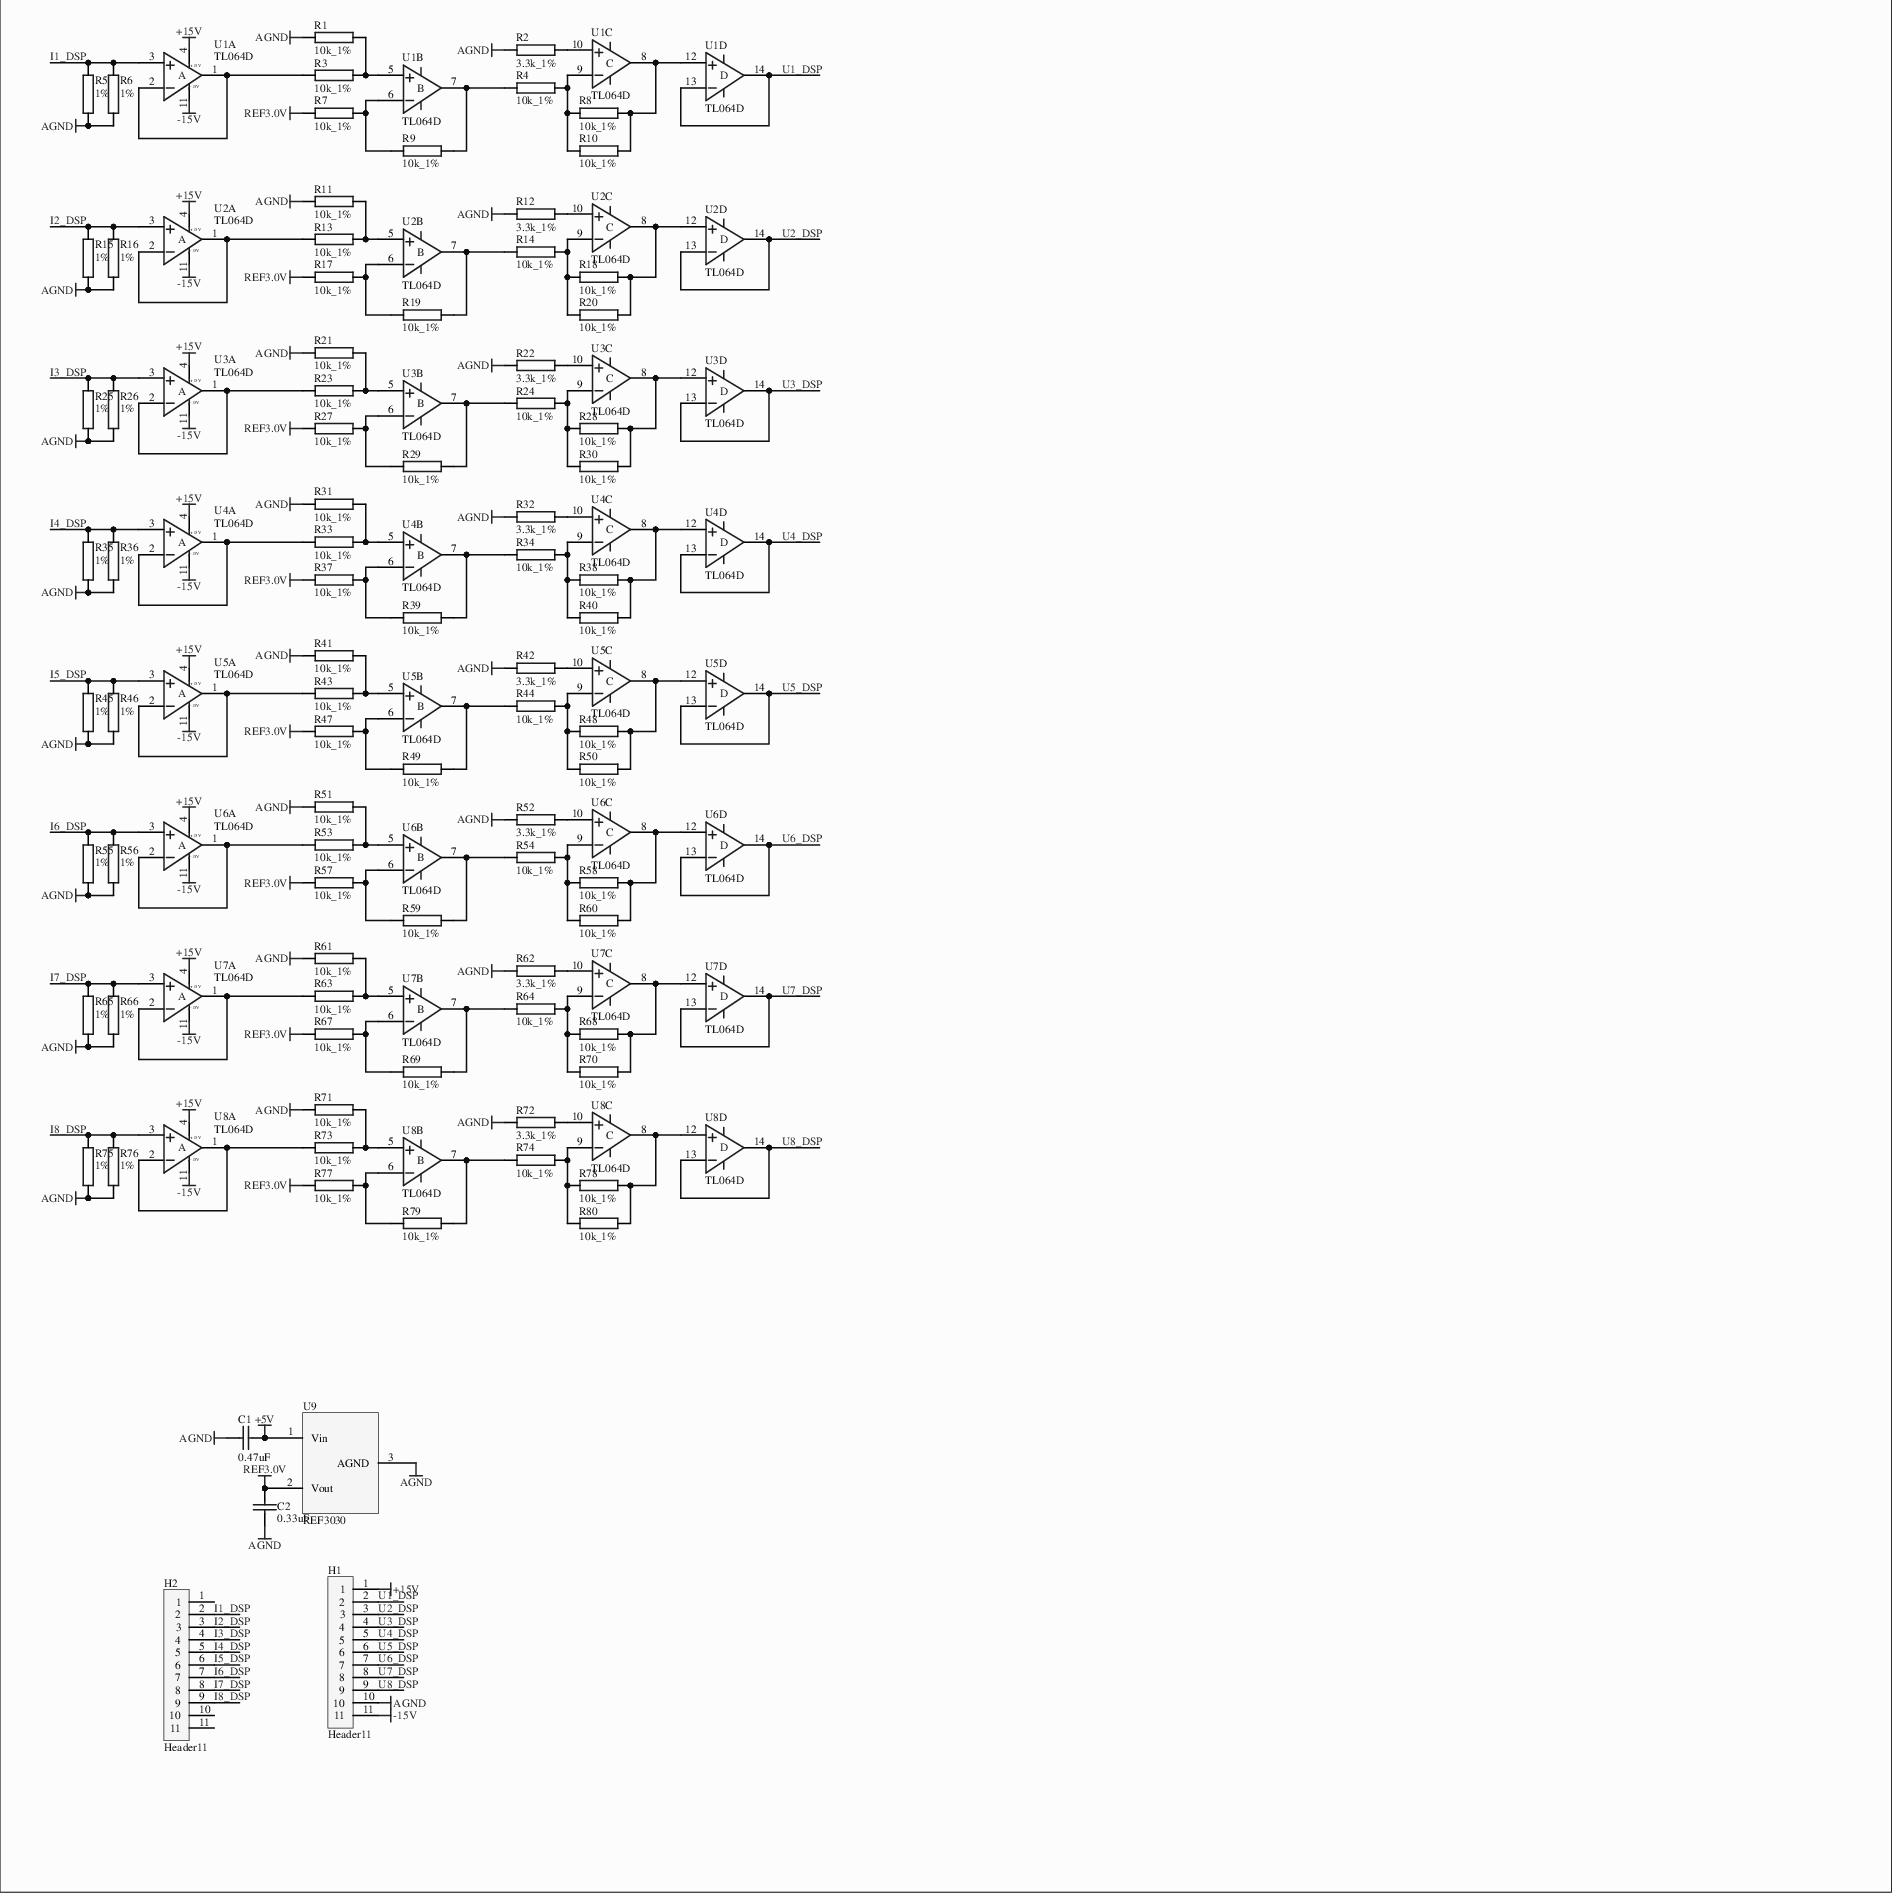
[diagram p0: MISC79030-3.SchDoc]
# Altium project MISC79030-2.PrjPcb
1 sheet, 93 parts. Net scope: global (net labels, ports and power ports of the same name join across sheets).
Board file: MISC79030.PcbDoc

## Sheet MISC79030-3.SchDoc
size 381 x 381 mm

### Parts
C1  0.47uF  [0603]
C2  0.33uF  [0603]
H1  Header11  [PinHeader11_1.27mm]
H2  Header11  [PinHeader11_1.27mm]
R1  10k_1%  [0603]
R2  3.3k_1%  [0603]
R3  10k_1%  [0603]
R4  10k_1%  [0603]
R5  1%  [0805]
R6  1%  [0805]
R7  10k_1%  [0603]
R8  10k_1%  [0603]
R9  10k_1%  [0603]
R10  10k_1%  [0603]
R11  10k_1%  [0603]
R12  3.3k_1%  [0603]
R13  10k_1%  [0603]
R14  10k_1%  [0603]
R15  1%  [0805]
R16  1%  [0805]
R17  10k_1%  [0603]
R18  10k_1%  [0603]
R19  10k_1%  [0603]
R20  10k_1%  [0603]
R21  10k_1%  [0603]
R22  3.3k_1%  [0603]
R23  10k_1%  [0603]
R24  10k_1%  [0603]
R25  1%  [0805]
R26  1%  [0805]
R27  10k_1%  [0603]
R28  10k_1%  [0603]
R29  10k_1%  [0603]
R30  10k_1%  [0603]
R31  10k_1%  [0603]
R32  3.3k_1%  [0603]
R33  10k_1%  [0603]
R34  10k_1%  [0603]
R35  1%  [0805]
R36  1%  [0805]
R37  10k_1%  [0603]
R38  10k_1%  [0603]
R39  10k_1%  [0603]
R40  10k_1%  [0603]
R41  10k_1%  [0603]
R42  3.3k_1%  [0603]
R43  10k_1%  [0603]
R44  10k_1%  [0603]
R45  1%  [0805]
R46  1%  [0805]
R47  10k_1%  [0603]
R48  10k_1%  [0603]
R49  10k_1%  [0603]
R50  10k_1%  [0603]
R51  10k_1%  [0603]
R52  3.3k_1%  [0603]
R53  10k_1%  [0603]
R54  10k_1%  [0603]
R55  1%  [0805]
R56  1%  [0805]
R57  10k_1%  [0603]
R58  10k_1%  [0603]
R59  10k_1%  [0603]
R60  10k_1%  [0603]
R61  10k_1%  [0603]
R62  3.3k_1%  [0603]
R63  10k_1%  [0603]
R64  10k_1%  [0603]
R65  1%  [0805]
R66  1%  [0805]
R67  10k_1%  [0603]
R68  10k_1%  [0603]
R69  10k_1%  [0603]
R70  10k_1%  [0603]
R71  10k_1%  [0603]
R72  3.3k_1%  [0603]
R73  10k_1%  [0603]
R74  10k_1%  [0603]
R75  1%  [0805]
R76  1%  [0805]
R77  10k_1%  [0603]
R78  10k_1%  [0603]
R79  10k_1%  [0603]
R80  10k_1%  [0603]
U1  TL064D  [TL064D_SOIC-14]  (parts A,B,C,D of 4)
U2  TL064D  [TL064D_SOIC-14]  (parts A,B,C,D of 4)
U3  TL064D  [TL064D_SOIC-14]  (parts A,B,C,D of 4)
U4  TL064D  [TL064D_SOIC-14]  (parts A,B,C,D of 4)
U5  TL064D  [TL064D_SOIC-14]  (parts A,B,C,D of 4)
U6  TL064D  [TL064D_SOIC-14]  (parts A,B,C,D of 4)
U7  TL064D  [TL064D_SOIC-14]  (parts A,B,C,D of 4)
U8  TL064D  [TL064D_SOIC-14]  (parts A,B,C,D of 4)
U9  REF3030  [SOT-23]

### Nets
+5V: C1.1 U9.1(Vin)
+15V: H1.1 U1.4 U2.4 U3.4 U4.4 U5.4 U6.4 U7.4 U8.4
-15V: H1.11 U1.11 U2.11 U3.11 U4.11 U5.11 U6.11 U7.11 U8.11
AGND: C1.2 C2.2 H1.10 R1.1 R2.1 R5.2 R6.2 R11.1 R12.1 R15.2 R16.2 R21.1 R22.1 R25.2 R26.2 R31.1 R32.1 R35.2 R36.2 R41.1 R42.1 R45.2 R46.2 R51.1 R52.1 R55.2 R56.2 R61.1 R62.1 R65.2 R66.2 R71.1 R72.1 R75.2 R76.2 U9.3(AGND)
REF3.0V: C2.1 R7.1 R17.1 R27.1 R37.1 R47.1 R57.1 R67.1 R77.1 U9.2(Vout)
I1_DSP: H2.2 R5.1 R6.1 U1.3
I2_DSP: H2.3 R15.1 R16.1 U2.3
I3_DSP: H2.4 R25.1 R26.1 U3.3
I4_DSP: H2.5 R35.1 R36.1 U4.3
I5_DSP: H2.6 R45.1 R46.1 U5.3
I6_DSP: H2.7 R55.1 R56.1 U6.3
I7_DSP: H2.8 R65.1 R66.1 U7.3
I8_DSP: H2.9 R75.1 R76.1 U8.3
U1_DSP: H1.2 U1.13 U1.14
U2_DSP: H1.3 U2.13 U2.14
U3_DSP: H1.4 U3.13 U3.14
U4_DSP: H1.5 U4.13 U4.14
U5_DSP: H1.6 U5.13 U5.14
U6_DSP: H1.7 U6.13 U6.14
U7_DSP: H1.8 U7.13 U7.14
U8_DSP: H1.9 U8.13 U8.14
NetR1_2: R1.2 R3.2 U1.5
NetR2_2: R2.2 U1.10
NetR3_1: R3.1 U1.1 U1.2
NetR4_1: R4.1 R9.2 U1.7
NetR4_2: R4.2 R8.1 R10.1 U1.9
NetR7_2: R7.2 R9.1 U1.6
NetR8_2: R8.2 R10.2 U1.8 U1.12
NetR11_2: R11.2 R13.2 U2.5
NetR12_2: R12.2 U2.10
NetR13_1: R13.1 U2.1 U2.2
NetR14_1: R14.1 R19.2 U2.7
NetR14_2: R14.2 R18.1 R20.1 U2.9
NetR17_2: R17.2 R19.1 U2.6
NetR18_2: R18.2 R20.2 U2.8 U2.12
NetR21_2: R21.2 R23.2 U3.5
NetR22_2: R22.2 U3.10
NetR23_1: R23.1 U3.1 U3.2
NetR24_1: R24.1 R29.2 U3.7
NetR24_2: R24.2 R28.1 R30.1 U3.9
NetR27_2: R27.2 R29.1 U3.6
NetR28_2: R28.2 R30.2 U3.8 U3.12
NetR31_2: R31.2 R33.2 U4.5
NetR32_2: R32.2 U4.10
NetR33_1: R33.1 U4.1 U4.2
NetR34_1: R34.1 R39.2 U4.7
NetR34_2: R34.2 R38.1 R40.1 U4.9
NetR37_2: R37.2 R39.1 U4.6
NetR38_2: R38.2 R40.2 U4.8 U4.12
NetR41_2: R41.2 R43.2 U5.5
NetR42_2: R42.2 U5.10
NetR43_1: R43.1 U5.1 U5.2
NetR44_1: R44.1 R49.2 U5.7
NetR44_2: R44.2 R48.1 R50.1 U5.9
NetR47_2: R47.2 R49.1 U5.6
NetR48_2: R48.2 R50.2 U5.8 U5.12
NetR51_2: R51.2 R53.2 U6.5
NetR52_2: R52.2 U6.10
NetR53_1: R53.1 U6.1 U6.2
NetR54_1: R54.1 R59.2 U6.7
NetR54_2: R54.2 R58.1 R60.1 U6.9
NetR57_2: R57.2 R59.1 U6.6
NetR58_2: R58.2 R60.2 U6.8 U6.12
NetR61_2: R61.2 R63.2 U7.5
NetR62_2: R62.2 U7.10
NetR63_1: R63.1 U7.1 U7.2
NetR64_1: R64.1 R69.2 U7.7
NetR64_2: R64.2 R68.1 R70.1 U7.9
NetR67_2: R67.2 R69.1 U7.6
NetR68_2: R68.2 R70.2 U7.8 U7.12
NetR71_2: R71.2 R73.2 U8.5
NetR72_2: R72.2 U8.10
NetR73_1: R73.1 U8.1 U8.2
NetR74_1: R74.1 R79.2 U8.7
NetR74_2: R74.2 R78.1 R80.1 U8.9
NetR77_2: R77.2 R79.1 U8.6
NetR78_2: R78.2 R80.2 U8.8 U8.12

Not connected (* = marked no-connect by the designer): H2 1 10 11

### Library data of the parts
C1 C2 = CAP: Capacitor
R1-R80 = ProE260.TMP_300K_25
U1-U8 = TL064D: TI TL064D